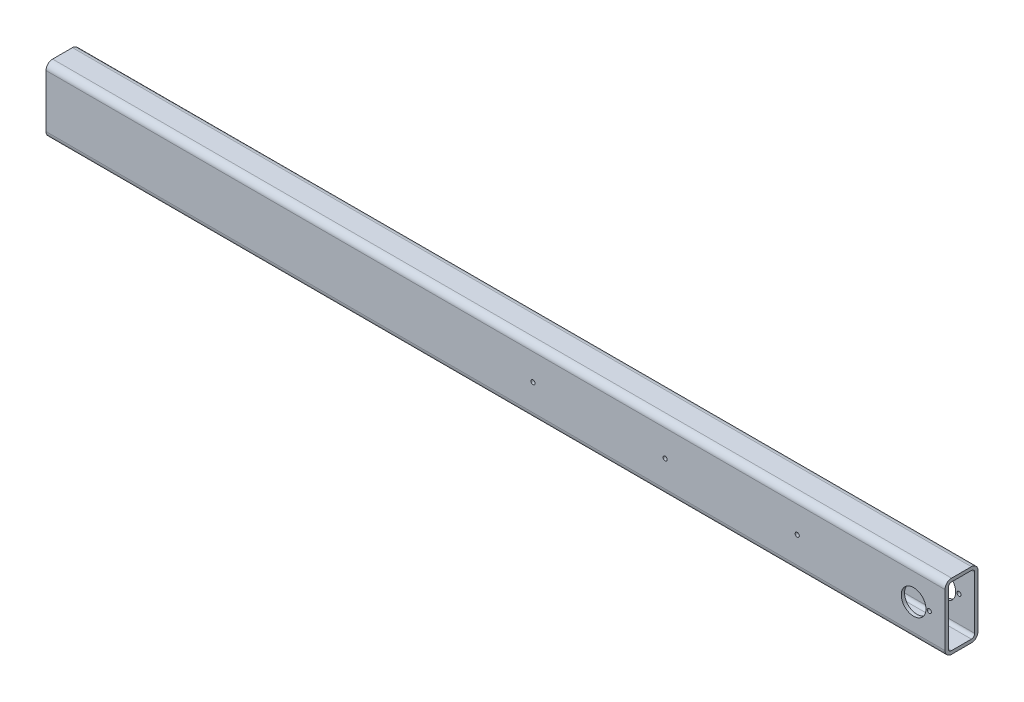
SolidWorks part; units mm, degrees
material "Q235A"
ref_plane "前视基准面" through (0, 0, 0) normal (0, 0, 1) x (1, 0, 0)
ref_plane "上视基准面" through (0, 0, 0) normal (0, 1, 0) x (1, 0, 0)
ref_plane "右视基准面" through (0, 0, 0) normal (1, 0, 0) x (0, 0, -1)
sketch "草图1" plane through (0, 0, 0) normal (0, 1, 0) x (1, 0, 0)
  line L0 (0, 0) -> (1089, 0)
  dimension "D1" = 1089
other "Gb／6728-1986矩形空心型钢 080 X 40 X 4(1)"
ref_plane "基准面1" through (0, 0, 0) normal (1, 0, 0) x (0, 0, -1)
sketch "Sketch12" plane through (0, 0, 0) normal (1, 0, 0) x (0, 0, -1)
  line L0 (-12, -36) -> (12, -36)
  line L1 (-16, -32) -> (-16, 32)
  line L2 (12, 36) -> (-12, 36)
  line L3 (16, 32) -> (16, -32)
  line L4 (-12, -40) -> (12, -40)
  line L5 (-20, -32) -> (-20, 32)
  line L6 (12, 40) -> (-12, 40)
  line L7 (20, 32) -> (20, -32)
  arc A0 (20, 32) -> (12, 40) centre (12, 32) ccw
  arc A1 (12, -40) -> (20, -32) centre (12, -32) ccw
  arc A2 (-20, -32) -> (-12, -40) centre (-12, -32) ccw
  arc A3 (-12, 40) -> (-20, 32) centre (-12, 32) ccw
  arc A4 (-12, 36) -> (-16, 32) centre (-12, 32) ccw
  arc A5 (16, 32) -> (12, 36) centre (12, 32) ccw
  arc A6 (12, -36) -> (16, -32) centre (12, -32) ccw
  arc A7 (-16, -32) -> (-12, -36) centre (-12, -32) ccw
  point P0 (0, 40)
  point P1 (20, 0)
  point P2 (0, -40)
  point P3 (-20, 0)
  point P4 (-20, 40)
  point P5 (20, 40)
  point P6 (20, -40)
  point P7 (-20, -40)
  point P8 (0, 0)
  point P33 (0, 0)
  dimension "D1" = 8
  dimension "Thickness" = 4
  dimension "V_leg" = 80
  dimension "H_leg" = 40
hole_wizard "M6 螺纹孔1" positions "草图2" profile "草图3" tap size "M6" standard "ISO" end condition through all
sketch "草图2" plane through (0, 0, -20) normal (0, 0, -1) x (-1, 0, 0)
  line L0 (-590, 0) -> (0, 0)
  line L2 (-590, 0) -> (-750, 0) construction
  point P0 (-590, 0)
  point P10 (-750, 0)
  point P11 (-910, 0)
  point P12 (-1070, 0)
  dimension "D1" = 590
  dimension "D3" = 160
  dimension "D2" = 4
sketch "草图3" plane through (590, 0, -20) normal (1, 0, 0) x (0, 1, 0)
  line L0 (0, 0) -> (0, 40)
  line L1 (0, 40) -> (2.5, 40)
  line L2 (2.5, 40) -> (2.5, 0)
  line L5 (2.5, 0) -> (0, 0)
  line L11 (0, -6.35) -> (0, 107.95) construction
  dimension "通孔螺纹孔钻头直径" = 5
  dimension "通孔螺纹孔钻头深度" = 40
cosmetic thread "孔螺蚊线1" parameters "D2"=6
cosmetic thread "孔螺蚊线2" parameters "D2"=6
cosmetic thread "孔螺蚊线3" parameters "D2"=6
cosmetic thread "孔螺蚊线4" parameters "D2"=6
sketch "草图4" plane through (0, 0, 20) normal (0, 0, 1) x (1, 0, 0)
  circle A0 centre (1051, 0) radius 15
  dimension "D1" = 30
extrude "切除-拉伸1" cut sketch "草图4" against normal through all
